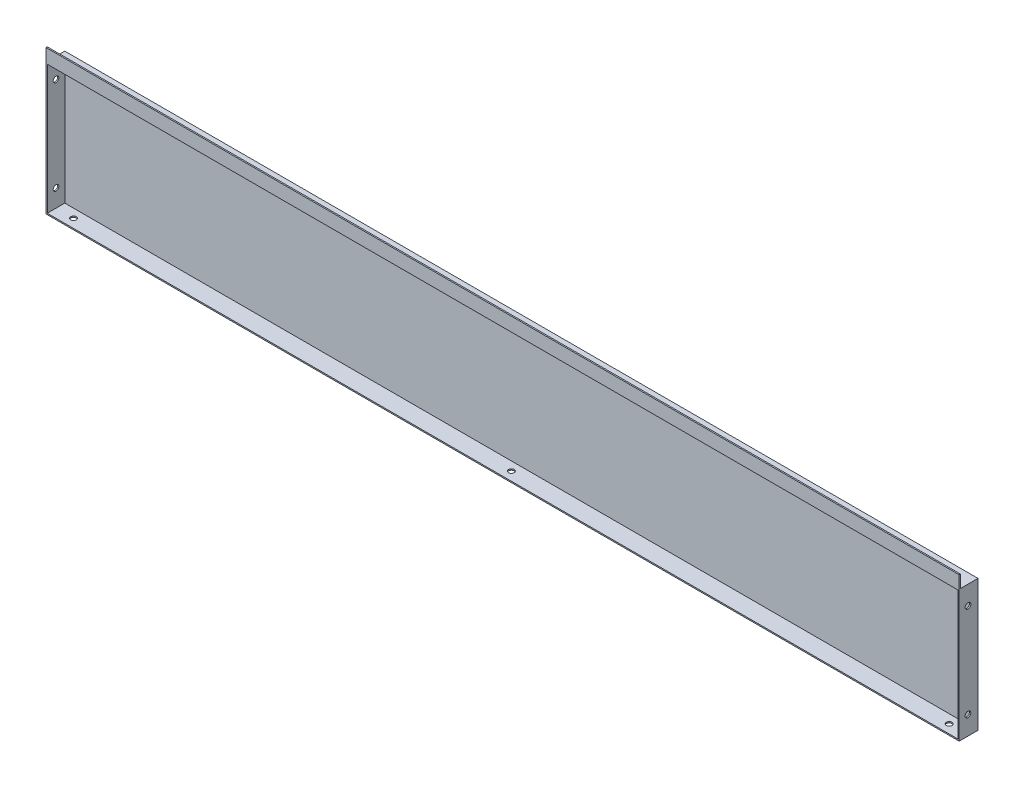
from build123d import *

# Parameters (mm, degrees)
SKETCH_1_W               = 1457
SKETCH_1_H               = 210
EXTRUDE_1_DEPTH          = 30
SHELL_1_T                = -2
SKETCH_2_W               = 1457
SKETCH_2_H               = 20
EXTRUDE_2_DEPTH          = 2
SKETCH_3_R               = 4.5
CUT_EXTRUDE_1_DEPTH      = 10
CUT_EXTRUDE_2_DEPTH      = 1525
CUT_EXTRUDE_2_DEPTH_BACK = 76
SKETCH_4_R               = 4.5


with BuildPart() as part:
    # 草图1 → 凸台-拉伸1 (new body)
    with BuildSketch(Plane.XY):
        with Locations((728.5, 105)):
            Rectangle(SKETCH_1_W, SKETCH_1_H)
    extrude(amount=EXTRUDE_1_DEPTH)

    # 抽壳1
    shell_1_openings = [part.faces().sort_by_distance(p)[0] for p in [
        (728.5, 105, 30),
    ]]
    offset(amount=SHELL_1_T, openings=shell_1_openings, kind=Kind.INTERSECTION)

    # 草图2 → 凸台-拉伸2 (add)
    with BuildSketch(Plane.XY.offset(30)):
        with Locations((728.5, 220)):
            Rectangle(SKETCH_2_W, SKETCH_2_H)
    extrude(amount=-EXTRUDE_2_DEPTH)

    # 草图3 → 切除-拉伸1 (cut)
    with BuildSketch(Plane(origin=(0, 2, 0), x_dir=(1, 0, 0), z_dir=(0, 1, 0))):
        with Locations(Location((1427, -16, 0), (0, 0, 270))):
            Circle(SKETCH_3_R)
        with Locations(Location((728.5, -16, 0), (0, 0, 270))):
            Circle(SKETCH_3_R)
        with Locations(Location((30, -16, 0), (0, 0, 270))):
            Circle(SKETCH_3_R)
    extrude(amount=-CUT_EXTRUDE_1_DEPTH, mode=Mode.SUBTRACT)

    # 草图4 → 切除-拉伸2 (cut, two sides: drawn at the far end of the back side and taken through both)
    with BuildSketch(Plane(origin=(2, 0, 0), x_dir=(0, 0, -1), z_dir=(1, 0, 0)).offset(-CUT_EXTRUDE_2_DEPTH_BACK)):
        with Locations(Location((-16, 30, 0), (0, 0, 180))):
            Circle(SKETCH_4_R)
        with Locations(Location((-16, 180, 0), (0, 0, 180))):
            Circle(SKETCH_4_R)
    extrude(amount=CUT_EXTRUDE_2_DEPTH + CUT_EXTRUDE_2_DEPTH_BACK, mode=Mode.SUBTRACT)


solid = part.part
